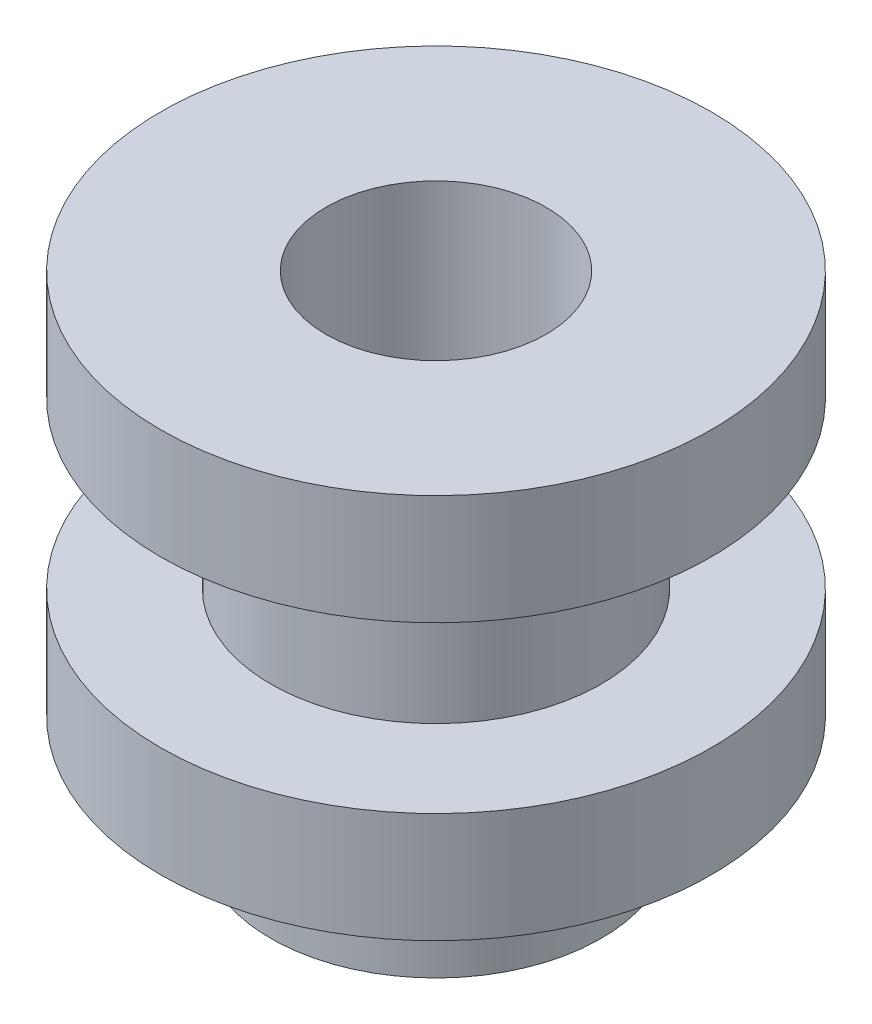
SolidWorks part; units mm, degrees
ref_plane "Front Plane" through (0, 0, 0) normal (0, 0, 1) x (1, 0, 0)
ref_plane "Top Plane" through (0, 0, 0) normal (0, 1, 0) x (1, 0, 0)
ref_plane "Right Plane" through (0, 0, 0) normal (1, 0, 0) x (0, 0, -1)
other "Configuration Table"
sketch "Sketch1" plane through (0, 0, 0) normal (0, 1, 0) x (1, 0, 0)
  circle A0 centre (0, 0) radius 5
  dimension "D1" = 10
extrude "Boss-Extrude1" add sketch "Sketch1" along normal blind 9
sketch "Sketch3" plane through (0, 0, 0) normal (0, 0, 1) x (1, 0, 0)
  line L0 (5, 0) -> (5, 9) construction
  line L1 (5, 7) -> (3, 7)
  line L2 (5, 7) -> (5, 4)
  line L3 (5, 4) -> (3, 4)
  line L4 (3, 7) -> (3, 4)
  line L5 (5, 9) -> (-5, 9) construction
  line L6 (5, 0) -> (3, 0)
  line L7 (5, 0) -> (5, 2)
  line L8 (5, 2) -> (3, 2)
  line L9 (3, 0) -> (3, 2)
  line L10 (0, 0) -> (0, 12.0002) construction
  dimension "D1" = 2
  dimension "D2" = 2
  dimension "D3" = 3
  dimension "D4" = 2
  dimension "D5" = 2
  dimension "D6" = 2
revolve "Cut-Revolve1" cut sketch "Sketch3" angle 360 about L10
sketch "Sketch4" plane through (0, 9, 0) normal (0, 1, 0) x (1, 0, 0)
  circle A0 centre (0, 0) radius 2
  dimension "D1" = 4
extrude "Cut-Extrude1" cut sketch "Sketch4" against normal through all
